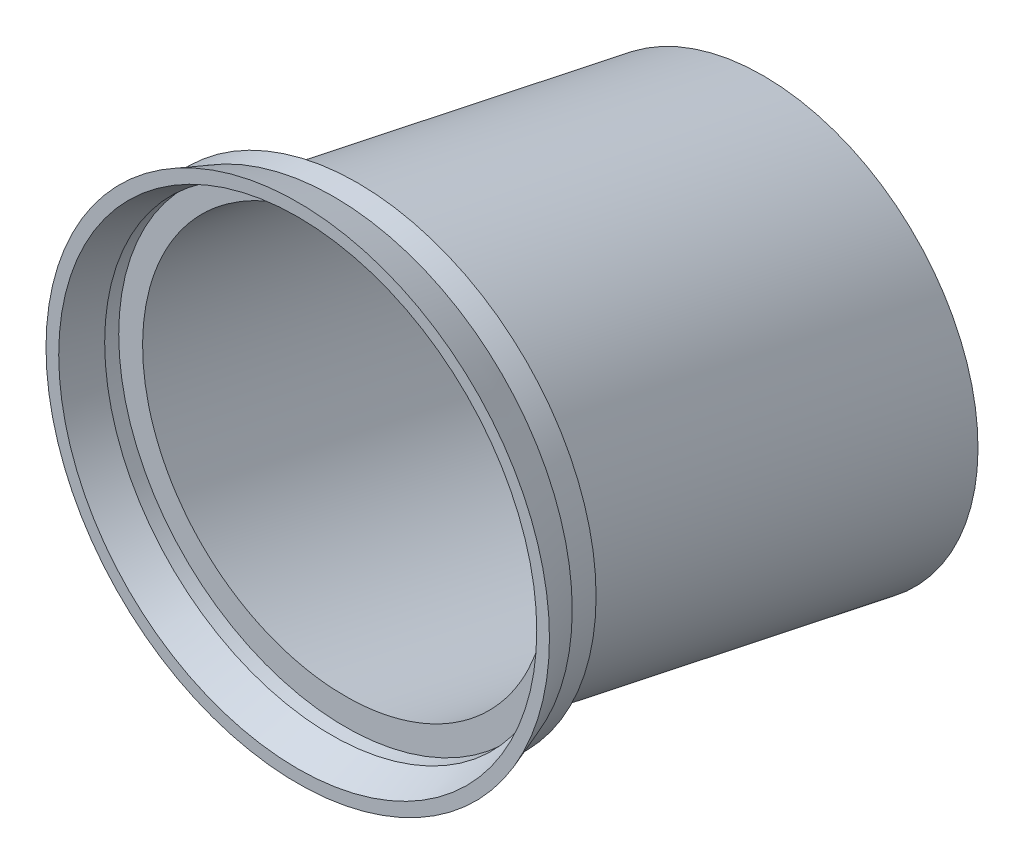
from build123d import *

# Parameters (mm, degrees)
SKETCH_1_R                = 20
EXTRUDE_1_DEPTH           = 3
EXTRUDE_1_TAPER           = -20
EXTRUDE_1_OTHER_WAY_DEPTH = 2
SKETCH_2_R                = 18
CUT_EXTRUDE_START         = 34
SKETCH_5_R                = 37.541334734
CUT_EXTRUDE_1_DEPTH       = 53
SHELL_1_T                 = -1


with BuildPart() as part:
    # 草图1 → 凸台-拉伸1 (new body)
    with BuildSketch(Plane.XY):
        Circle(SKETCH_1_R)
    extrude(amount=EXTRUDE_1_DEPTH, taper=EXTRUDE_1_TAPER)

    # 草图1 → 凸台-拉伸1 other way (add)
    with BuildSketch(Plane.XY):
        Circle(SKETCH_1_R)
    extrude(amount=-EXTRUDE_1_OTHER_WAY_DEPTH)

    # 扫描1: sweep along a path in 草图3
    with BuildLine(Plane(origin=(0, 0, 0), x_dir=(0, 0, -1), z_dir=(1, 0, 0))) as sweep_1_path:
        Line((2, 0), (46.016642033, -9.356026087))
    # 草图2 → 扫描1 (sweep)
    with BuildSketch(Plane(origin=(0, 0, -2), x_dir=(-1, 0, 0), z_dir=(0, 0, -1))):
        Circle(SKETCH_2_R)
    sweep(path=sweep_1_path.line)

    # 草图5 → 切除-拉伸1 (cut)
    with BuildSketch(Plane(origin=(0, 0, -2), x_dir=(-1, 0, 0), z_dir=(0, 0, -1)).offset(CUT_EXTRUDE_START)):
        Circle(SKETCH_5_R)
    extrude(amount=CUT_EXTRUDE_1_DEPTH, mode=Mode.SUBTRACT)

    # 抽壳1
    shell_1_openings = [part.faces().sort_by_distance(p)[0] for p in [
        (0, 0, 3),
        (-1.512e-06, -7.226932051, -36),
    ]]
    offset(amount=SHELL_1_T, openings=shell_1_openings, kind=Kind.INTERSECTION)


solid = part.part
